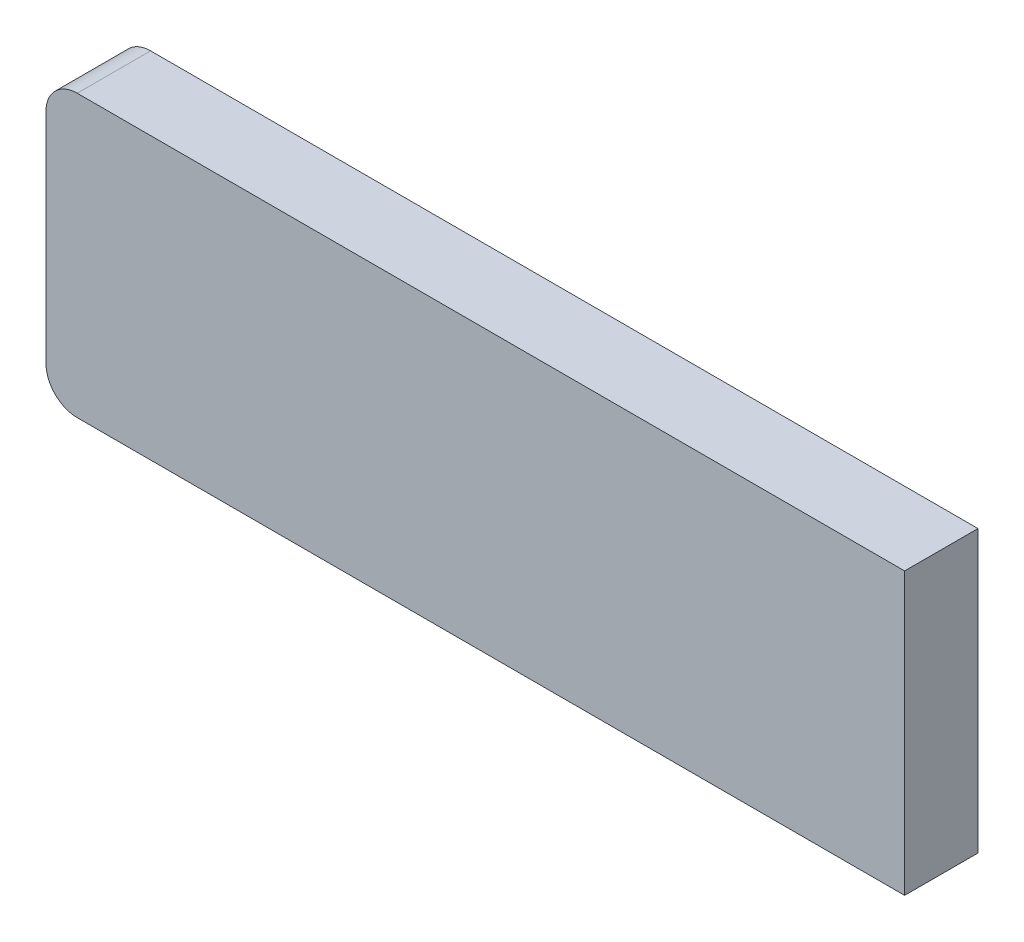
from build123d import *

# Parameters (mm, degrees)
EXTRUDE_1_DEPTH = 23.5


with BuildPart() as part:
    # 草图1 → 凸台-拉伸1 (new body)
    with BuildSketch(Plane.XY):
        with BuildLine():
            Line((-132.5, -45), (132.5, -45))
            Line((132.5, -45), (132.5, 45))
            Line((132.5, 45), (-132.5, 45))
            ThreePointArc((-132.5, 45), (-139.571067812, 42.071067812), (-142.5, 35))
            Line((-142.5, 35), (-142.5, -35))
            ThreePointArc((-142.5, -35), (-139.571067812, -42.071067812), (-132.5, -45))
        make_face()
    extrude(amount=EXTRUDE_1_DEPTH)


solid = part.part
